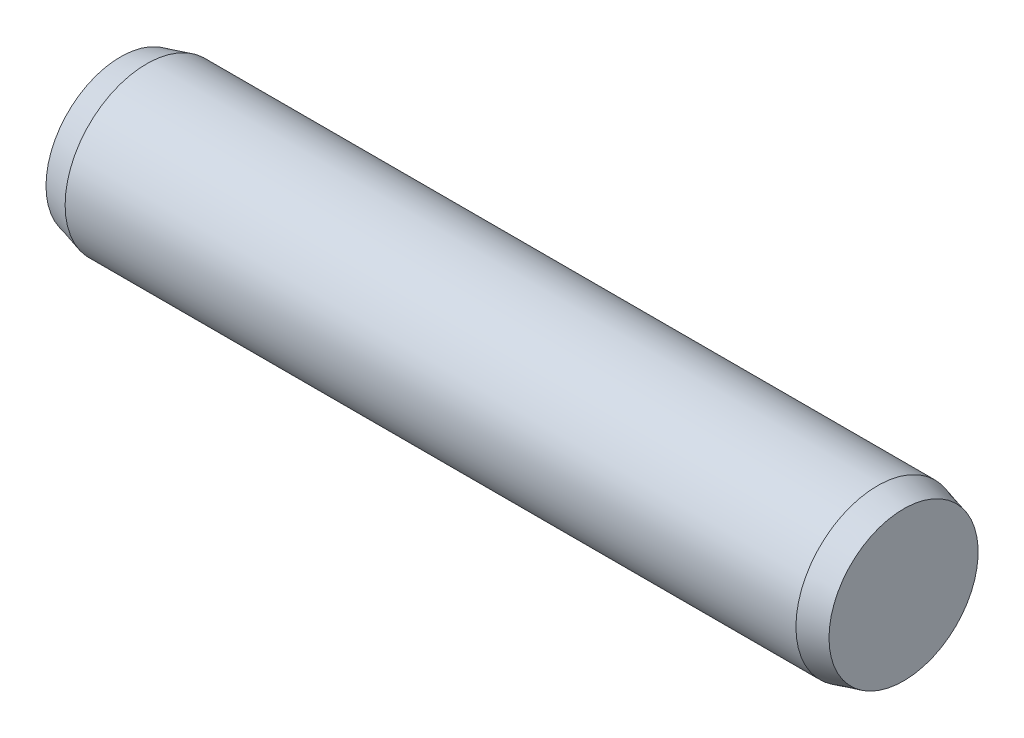
SolidWorks part; units mm, degrees
material "35钢"
ref_plane "Front" through (0, 0, 0) normal (0, 0, 1) x (1, 0, 0)
ref_plane "Top" through (0, 0, 0) normal (0, 1, 0) x (1, 0, 0)
ref_plane "Right" through (0, 0, 0) normal (1, 0, 0) x (0, 0, -1)
sketch "Sketch1" plane through (0, 0, 0) normal (0, 0, 1) x (1, 0, 0)
  line L0 (0, 0) -> (0.482, 0) construction
  line L1 (-1.4, 0) -> (10.6, 0)
  line L2 (-1, 1.25) -> (10.2, 1.25)
  line L3 (10.6, 1.1428) -> (10.6, 0)
  line L4 (10.2, 1.25) -> (10.6, 1.1428)
  line L5 (-1, -1.25) -> (10.2, -1.25) construction
  line L6 (-1, 1.25) -> (-1.4, 1.1428)
  line L7 (-1.4, 1.1428) -> (-1.4, 0)
  point P13 (4.6, 1.25)
revolve "Base-Revolve" add sketch "Sketch1" angle 360 about L0
equation "\"D2@Sketch1\" = \"c@Sketch1\""
